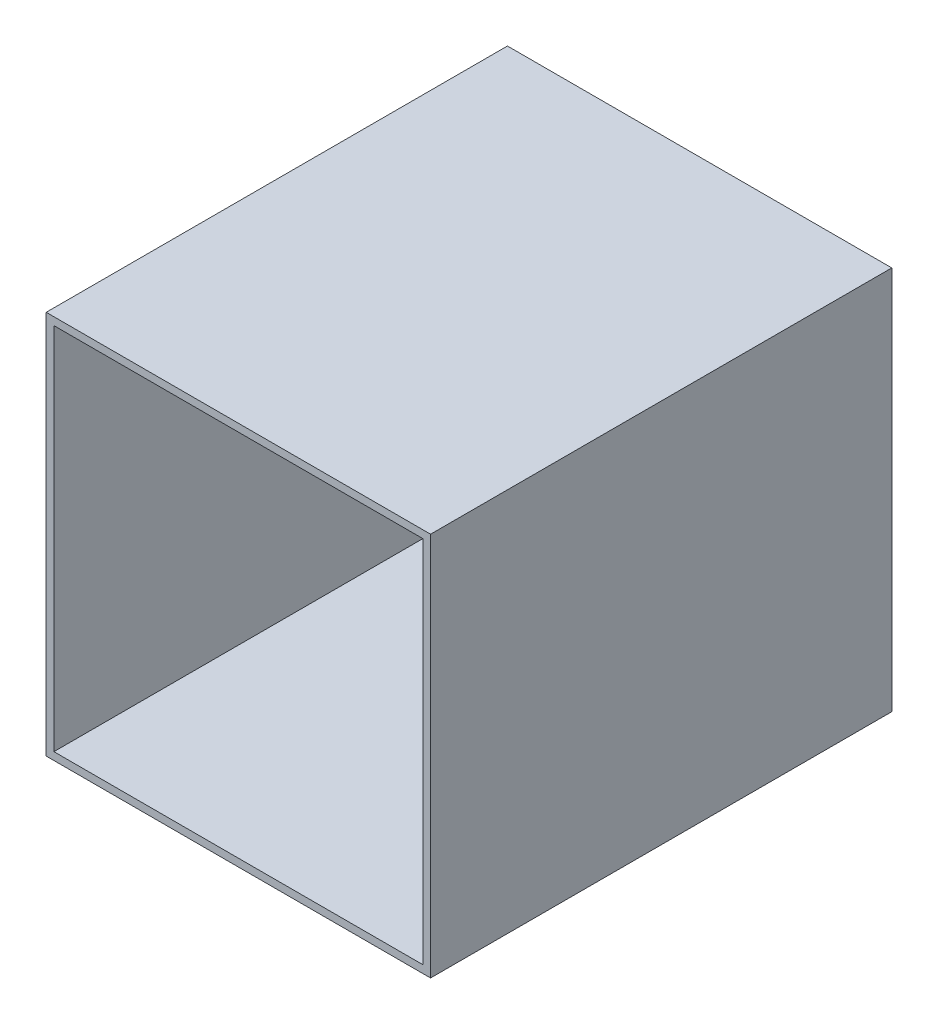
from build123d import *

# Parameters (mm, degrees)
SKETCH1_W           = 500
SKETCH1_H           = 500
BOSS_EXTRUDE1_DEPTH = 600
SHELL1_T            = -10


with BuildPart() as part:
    # Sketch1 → Boss-Extrude1 (new body)
    with BuildSketch(Plane.XY):
        with Locations((250, 250)):
            Rectangle(SKETCH1_W, SKETCH1_H)
    extrude(amount=BOSS_EXTRUDE1_DEPTH)

    # Shell1
    shell1_openings = [part.faces().sort_by_distance(p)[0] for p in [
        (250, 250, 600),
    ]]
    offset(amount=SHELL1_T, openings=shell1_openings, kind=Kind.INTERSECTION)


solid = part.part
